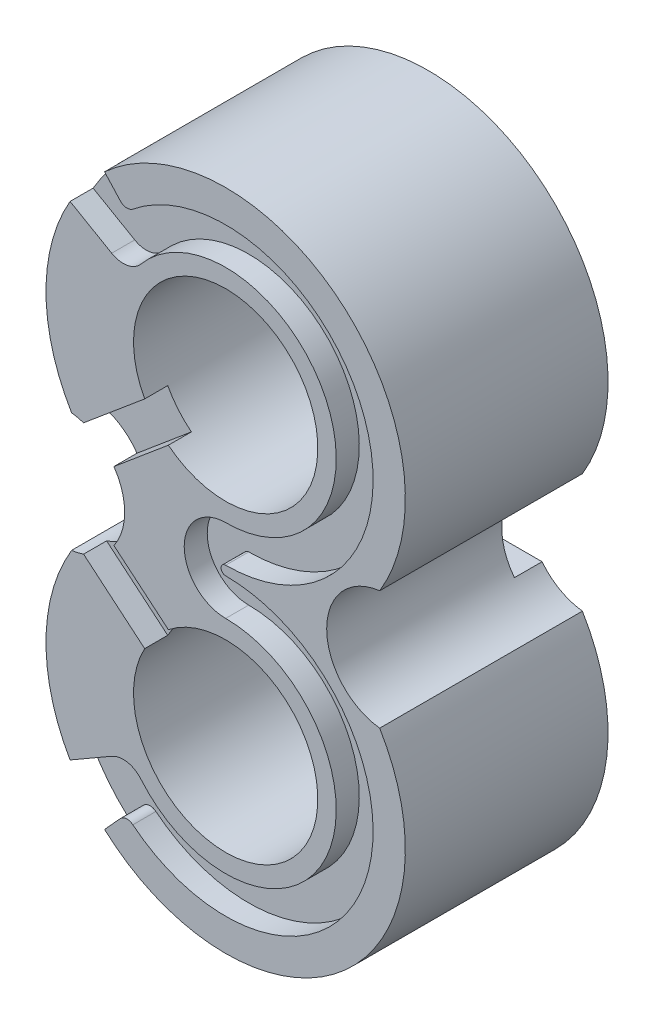
from build123d import *

# Parameters (mm, degrees)
SKETCH_1_R             = 10
EXTRUDE_1_DEPTH        = 22
CUT_EXTRUDE_1_DEPTH    = 2.5
FILLET_1_R             = 1
FILLET_2_R             = 2.5
FILLET_1_OF_MIRROR_1_R = 1
FILLET_2_OF_MIRROR_1_R = 2.5
CUT_EXTRUDE_2_DEPTH    = 2.5
CUT_EXTRUDE_3_DEPTH    = 1.5
SKETCH_5_W             = 15.539550215
SKETCH_5_H             = 8
CUT_EXTRUDE_4_DEPTH    = 1.5
SKETCH_6_W             = 13.998675607
SKETCH_6_H             = 8
CUT_EXTRUDE_5_DEPTH    = 3
FILLET_3_R             = 1


with BuildPart() as part:
    # 草图1 → 凸台-拉伸1 (new body)
    with BuildSketch(Plane.XY):
        with BuildLine():
            ThreePointArc((16.714762364, 6.456757539), (0, 36), (-16.714762364, 6.456757539))
            ThreePointArc((-16.714762364, 6.456757539), (-10.963282289, 0), (-16.714762364, -6.456757539))
            ThreePointArc((-16.714762364, -6.456757539), (0, -36), (16.714762364, -6.456757539))
            ThreePointArc((16.714762364, -6.456757539), (10.963282289, 0), (16.714762364, 6.456757539))
        make_face()
        with Locations((0, 16.5)):
            Circle(SKETCH_1_R, mode=Mode.SUBTRACT)
        with Locations((0, -16.5)):
            Circle(SKETCH_1_R, mode=Mode.SUBTRACT)
    extrude(amount=EXTRUDE_1_DEPTH)

    # 草图2 → 切除-拉伸1 (cut)
    with BuildSketch(Plane.XY.offset(22)):
        with BuildLine():
            Line((-10.392304845, 22.5), (-20.279992845, 28.208659328))
            Line((-20.279992845, 28.208659328), (-16.120486586, 34.166566083))
            Line((-16.120486586, 34.166566083), (-10.784713231, 28.319050745))
            ThreePointArc((-10.784713231, 28.319050745), (14.918190439, 22.283389494), (0, 0.5))
            ThreePointArc((0, 0.5), (-0.353553391, 0.353553391), (-0.5, 0))
            Line((-0.5, 0), (-4.5, 0))
            ThreePointArc((-4.5, 0), (-3.181980515, 3.181980515), (0, 4.5))
            ThreePointArc((0, 4.5), (10.392304845, 22.5), (-10.392304845, 22.5))
        make_face()
    cut_extrude_1 = extrude(amount=-CUT_EXTRUDE_1_DEPTH, mode=Mode.SUBTRACT)

    # 圆角1
    fillet_1_edges = [part.edges().sort_by_distance(p)[0] for p in [
        (-10.784713231, 28.319050745, 20.75),
    ]]
    fillet(fillet_1_edges, radius=FILLET_1_R)

    # 圆角2
    fillet_2_edges = [part.edges().sort_by_distance(p)[0] for p in [
        (-10.392304845, 22.5, 20.75),
    ]]
    fillet(fillet_2_edges, radius=FILLET_2_R)

    # 镜向1: 切除-拉伸1 across plane
    add(cut_extrude_1.mirror(Plane.ZX), mode=Mode.SUBTRACT)

    # 圆角1 of 镜向1
    fillet_1_of_mirror_1_edges = [part.edges().sort_by_distance(p)[0] for p in [
        (-10.784713231, -28.319050745, 20.75),
    ]]
    fillet(fillet_1_of_mirror_1_edges, radius=FILLET_1_OF_MIRROR_1_R)

    # 圆角2 of 镜向1
    fillet_2_of_mirror_1_edges = [part.edges().sort_by_distance(p)[0] for p in [
        (-10.392304845, -22.5, 20.75),
    ]]
    fillet(fillet_2_of_mirror_1_edges, radius=FILLET_2_OF_MIRROR_1_R)

    # 草图3 → 切除-拉伸2 (cut)
    with BuildSketch(Plane.XY.offset(22)):
        Polygon((-7.454777322, 12.855513677), (-16.290741775, 5.441259163), (-13.719591337, 2.377081391), (-4.883626883, 9.791335905), align=None)
        Polygon((-13.453227562, -2.600587136), (-5.167237951, -9.553357963), (-7.738388389, -12.617535735), (-16.448259291, -5.309086274), align=None)
    extrude(amount=-CUT_EXTRUDE_2_DEPTH, mode=Mode.SUBTRACT)

    # 草图4 → 切除-拉伸3 (cut)
    with BuildSketch(Plane(origin=(0, 0, 0), x_dir=(-1, 0, 0), z_dir=(0, 0, -1))):
        Polygon((3, 14.697418143), (16.714762364, 6.456757539), (16.714762364, -6.456757539), (3, -14.697418143), align=None)
    extrude(amount=-CUT_EXTRUDE_3_DEPTH, mode=Mode.SUBTRACT)

    # 草图5 → 切除-拉伸4 (cut)
    with BuildSketch(Plane(origin=(0, 0, 1.5), x_dir=(-1, 0, 0), z_dir=(0, 0, -1))):
        with Locations((10.769775108, 0)):
            Rectangle(SKETCH_5_W, SKETCH_5_H)
    extrude(amount=-CUT_EXTRUDE_4_DEPTH, mode=Mode.SUBTRACT)

    # 草图6 → 切除-拉伸5 (cut)
    with BuildSketch(Plane(origin=(0, 0, 0), x_dir=(-1, 0, 0), z_dir=(0, 0, -1))):
        with Locations((-7.999337804, 0)):
            Rectangle(SKETCH_6_W, SKETCH_6_H)
    extrude(amount=-CUT_EXTRUDE_5_DEPTH, mode=Mode.SUBTRACT)

    # 圆角3
    fillet_3_edges = [part.edges().sort_by_distance(p)[0] for p in [
        (-3, 4, 2.25),
        (-3, -4, 2.25),
        (1, 4, 1.5),
        (1, -4, 1.5),
    ]]
    fillet(fillet_3_edges, radius=FILLET_3_R)


solid = part.part
